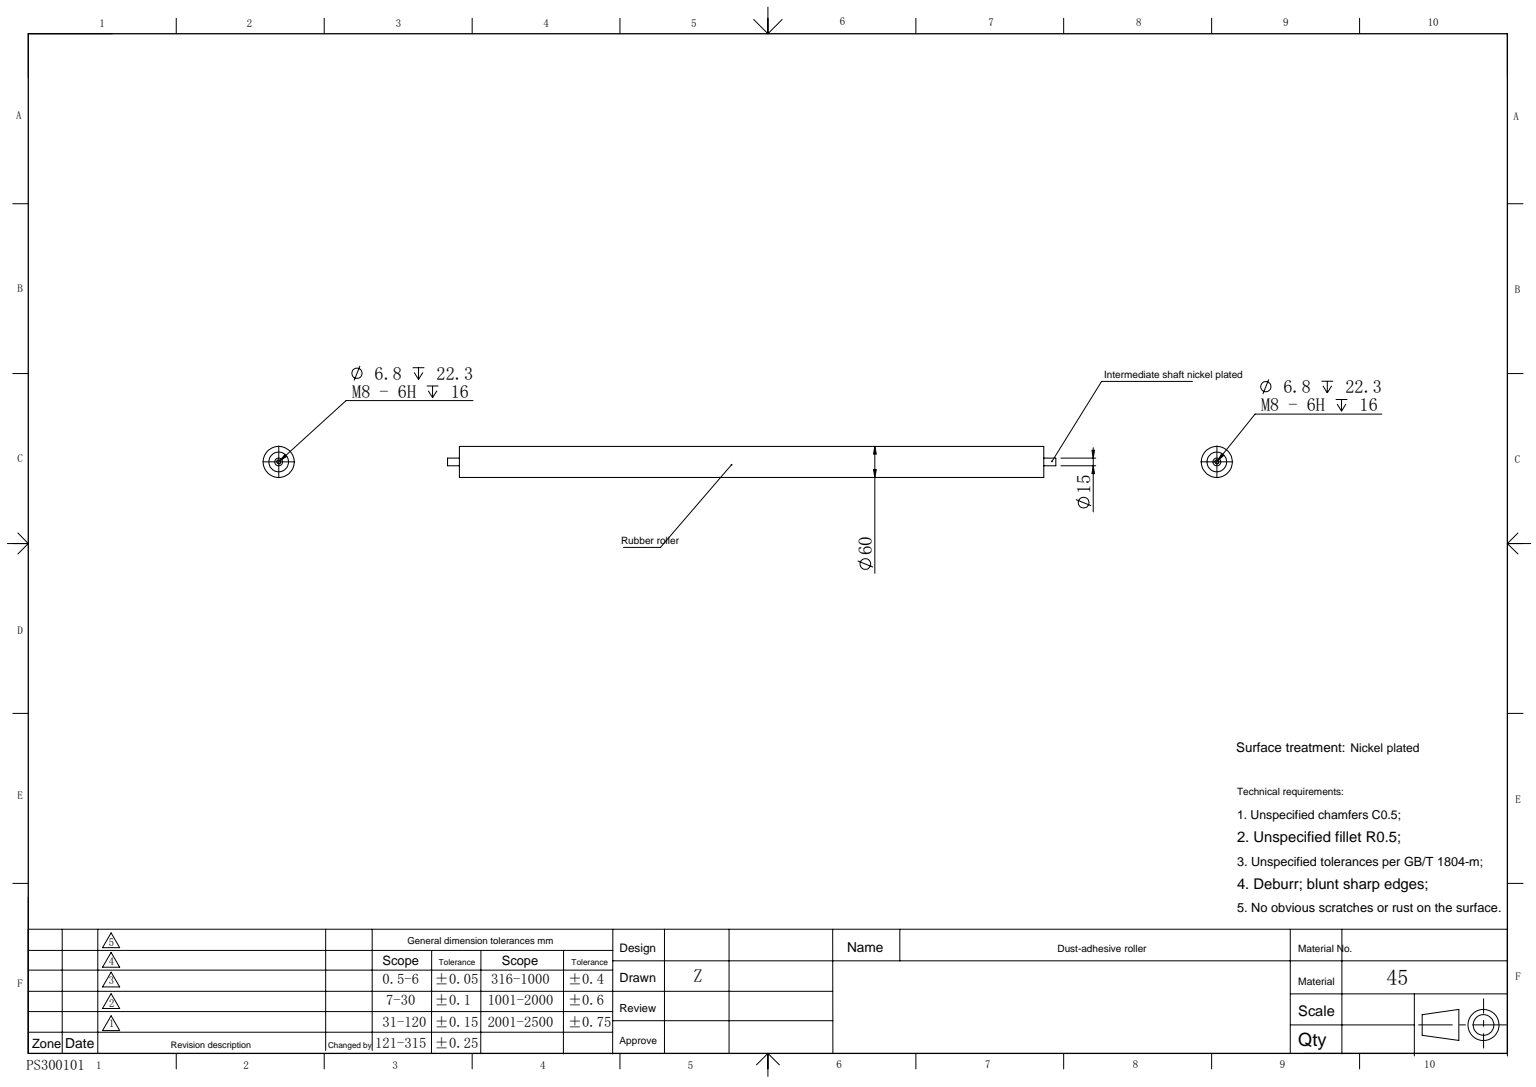
from build123d import *

# Parameters (mm, degrees)
SKETCH_1_R      = 7.5
EXTRUDE_1_DEPTH = 588
SKETCH_2_R      = 19
EXTRUDE_2_DEPTH = 550
SKETCH_3_R      = 30
SKETCH_3_R_2    = 19
EXTRUDE_3_DEPTH = 565


with BuildPart() as part:
    # 草图1 → 凸台-拉伸1 (new, symmetric)
    with BuildSketch(Plane.XY):
        Circle(SKETCH_1_R)
    extrude(amount=EXTRUDE_1_DEPTH, both=True)

    # 草图2 → 凸台-拉伸2 (add, symmetric)
    with BuildSketch(Plane.XY):
        Circle(SKETCH_2_R)
    extrude(amount=EXTRUDE_2_DEPTH, both=True)

    # 草图5 → M8 螺纹孔1 (revolve, cut)
    with BuildSketch(Plane(origin=(0, 0, -588), x_dir=(0, 1, 0), z_dir=(1, 0, 0))):
        Polygon((0, 0), (0, 24.292926105), (3.4, 22.25), (3.4, 0), align=None)
    revolve(axis=Axis((0, 0, -594.35), (0, 0, 1)), mode=Mode.SUBTRACT)

    # 草图8 → M8 螺纹孔2 (revolve, cut)
    with BuildSketch(Plane(origin=(0, 0, 588), x_dir=(0, -1, 0), z_dir=(1, 0, 0))):
        Polygon((0, 0), (0, 24.292926105), (3.4, 22.25), (3.4, 0), align=None)
    revolve(axis=Axis((0, 0, 594.35), (0, 0, -1)), mode=Mode.SUBTRACT)


with BuildPart() as body_2:
    # 草图3 → 凸台-拉伸3 (new, symmetric)
    with BuildSketch(Plane.XY):
        Circle(SKETCH_3_R)
        Circle(SKETCH_3_R_2, mode=Mode.SUBTRACT)
    extrude(amount=EXTRUDE_3_DEPTH, both=True)


solid = Compound([part.part, body_2.part])
